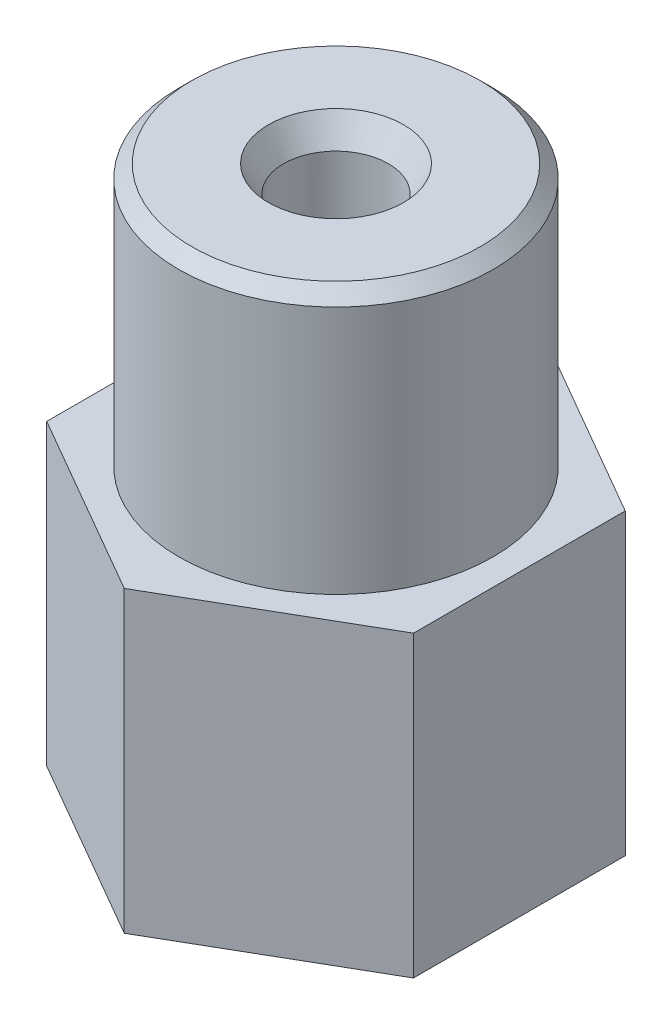
SolidWorks part; units mm, degrees
material "Copper"
ref_plane "Front Plane" through (0, 0, 0) normal (0, 0, 1) x (1, 0, 0)
ref_plane "Top Plane" through (0, 0, 0) normal (0, 1, 0) x (1, 0, 0)
ref_plane "Right Plane" through (0, 0, 0) normal (1, 0, 0) x (0, 0, -1)
sketch "Sketch1" plane through (0, 0, 0) normal (0, 0, 1) x (1, 0, 0)
  line L0 (0, 0) -> (0, 12.5) construction
  line L1 (0.2, 0) -> (0.375, 0)
  line L2 (0.375, 0) -> (1.4142, 1.8)
  line L3 (1.4142, 1.8) -> (2.5, 1.8)
  line L6 (2.5, 1.8) -> (2.5, 6.5)
  line L7 (2.5, 6.5) -> (3, 7.366)
  line L8 (3, 7.366) -> (3, 12.25)
  line L9 (2.75, 12.5) -> (1.2887, 12.5)
  line L10 (0.2, 0) -> (0.2, 0.6)
  line L11 (0.2, 0.6) -> (0.5, 1.1196)
  line L12 (0.5, 1.1196) -> (0.5, 3.1196)
  line L13 (0.5, 3.1196) -> (1, 3.9856)
  line L14 (1, 3.9856) -> (1, 12)
  line L15 (1, 12) -> (1.2887, 12.5)
  line L16 (3, 12.25) -> (2.75, 12.5)
  point P3 (3, 12.5)
  dimension "D1" = 12.5
  dimension "D2" = 120
  dimension "D3" = 5
  dimension "D4" = 10.7
  dimension "D5" = 6
  dimension "D6" = 0.75
  dimension "D7" = 2
  dimension "D8" = 0.4
  dimension "D9" = 1
  dimension "D10" = 0.6
  dimension "D11" = 60
  dimension "D12" = 60
  dimension "D13" = 0.5
  dimension "D14" = 6
  dimension "D15" = 2
revolve "Revolve1" add sketch "Sketch1" angle 360 about L0
sketch "Sketch2" plane through (0, 1.8, 0) normal (0, -1, 0) x (1, 0, 0)
  line L1 (0, 4.0415) -> (-3.5, 2.0207)
  line L2 (-3.5, 2.0207) -> (-3.5, -2.0207)
  line L3 (-3.5, -2.0207) -> (0, -4.0415)
  line L4 (0, -4.0415) -> (3.5, -2.0207)
  line L5 (3.5, -2.0207) -> (3.5, 2.0207)
  line L6 (3.5, 2.0207) -> (0, 4.0415)
  circle A0 centre (0, 0) radius 3.5 construction
  dimension "D1" = 7
extrude "Boss-Extrude1" add sketch "Sketch2" against normal offset from surface (5.7 mm away) 5 up to face at (0, 12.5, -1.2887)
